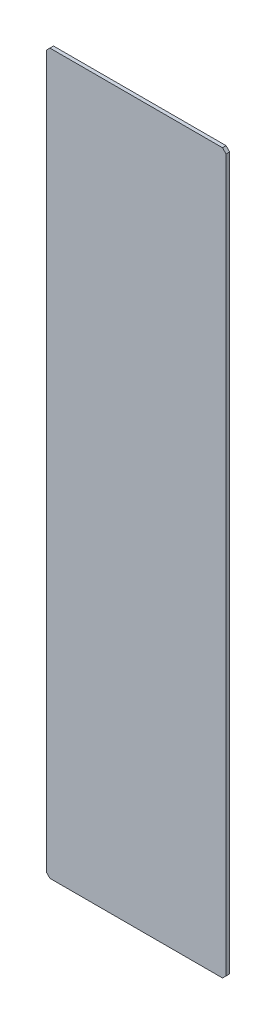
from build123d import *

# Parameters (mm, degrees)
SKETCH_1_W      = 500
SKETCH_1_H      = 2000
EXTRUDE_1_DEPTH = 5
CHAMFER_1_SIZE  = 10


with BuildPart() as part:
    # 草图1 → 凸台-拉伸1 (new, symmetric)
    with BuildSketch(Plane.XY):
        Rectangle(SKETCH_1_W, SKETCH_1_H)
    extrude(amount=EXTRUDE_1_DEPTH, both=True)

    # 倒角1
    chamfer_1_edges = [part.edges().sort_by_distance(p)[0] for p in [
        (250, -1000, 0),
        (-250, -1000, 0),
        (-250, 1000, 0),
        (250, 1000, 0),
    ]]
    chamfer(chamfer_1_edges, length=CHAMFER_1_SIZE)


solid = part.part
